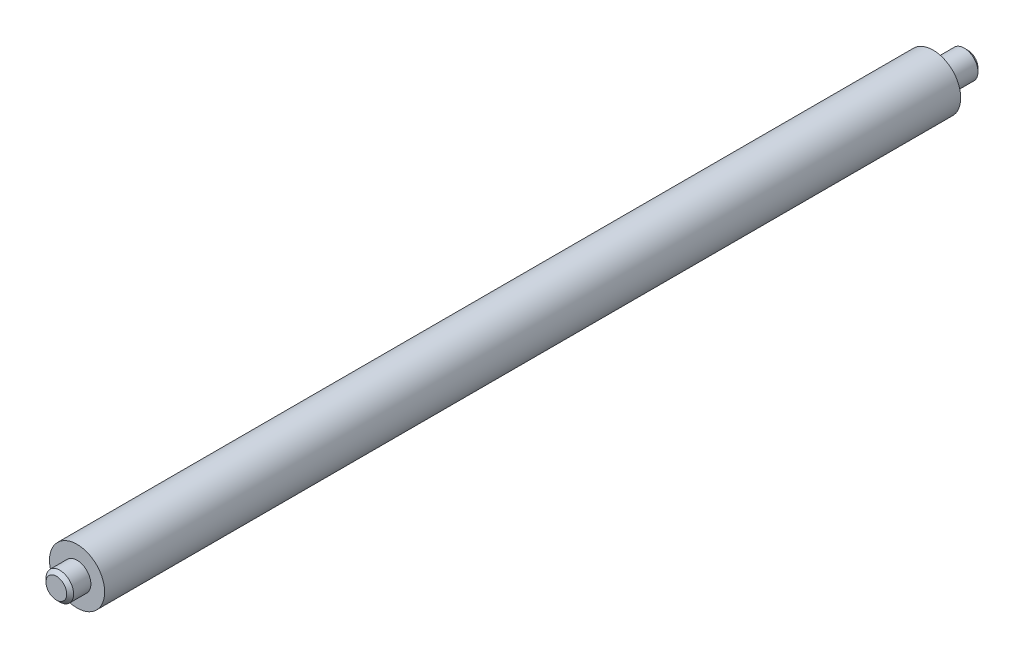
SolidWorks part; units mm, degrees
ref_plane "Front Plane" through (0, 0, 0) normal (0, 0, 1) x (1, 0, 0)
ref_plane "Top Plane" through (0, 0, 0) normal (0, 1, 0) x (1, 0, 0)
ref_plane "Right Plane" through (0, 0, 0) normal (1, 0, 0) x (0, 0, -1)
sketch "Sketch1" plane through (0, 0, 0) normal (0, 0, 1) x (1, 0, 0)
  circle A0 centre (0, 0) radius 8
  dimension "D1" = 16
extrude "Boss-Extrude1" add sketch "Sketch1" along normal blind 248
sketch "Sketch2" plane through (0, 0, 0) normal (0, 0, -1) x (-1, 0, 0)
  circle A0 centre (0, 0) radius 4
  dimension "D1" = 8
extrude "Boss-Extrude2" add sketch "Sketch2" along normal blind 10
sketch "Sketch3" plane through (0, 0, 248) normal (0, 0, 1) x (1, 0, 0)
  circle A0 centre (0, 0) radius 4
  dimension "D1" = 8
extrude "Boss-Extrude3" add sketch "Sketch3" along normal blind 6
sketch "Sketch4" plane through (0, 0, 0) normal (0, 0, -1) x (-1, 0, 0)
  circle A0 centre (0, 0) radius 8 construction
  circle A1 centre (0, 0) radius 8
curve "Helix/Spiral1" pitch 6.6471 height 621.5 turns 93.5
ref_plane "Plane1" through (5.6569, 5.6569, 0) normal (-0.701, 0.701, 0.1311) x (0.7128, 0.6945, 0.0977)
sketch "Sketch5" plane through (5.6569, 5.6569, 0) normal (-0.701, 0.701, 0.1311) x (0.7128, 0.6945, 0.0977)
  line L0 (0, 2.5) -> (-3.6784, 0)
  line L1 (0, 2.5) -> (3.6784, 2.5)
  line L3 (0, -2.5) -> (3.6784, -2.5)
  line L4 (3.6784, 2.5) -> (3.6784, -2.5)
  line L5 (-1.8392, 1.25) -> (3.6784, -2.5) construction
  line L6 (-1.8392, -1.25) -> (3.6784, 2.5) construction
  line L7 (-3.6784, 0) -> (0, -2.5)
  point P0 (0, 0)
  dimension "D1" = 5
chamfer "Chamfer1" distance 1 angle 45 2 edges at (-4, 0, -10) (4, 0, 254)
